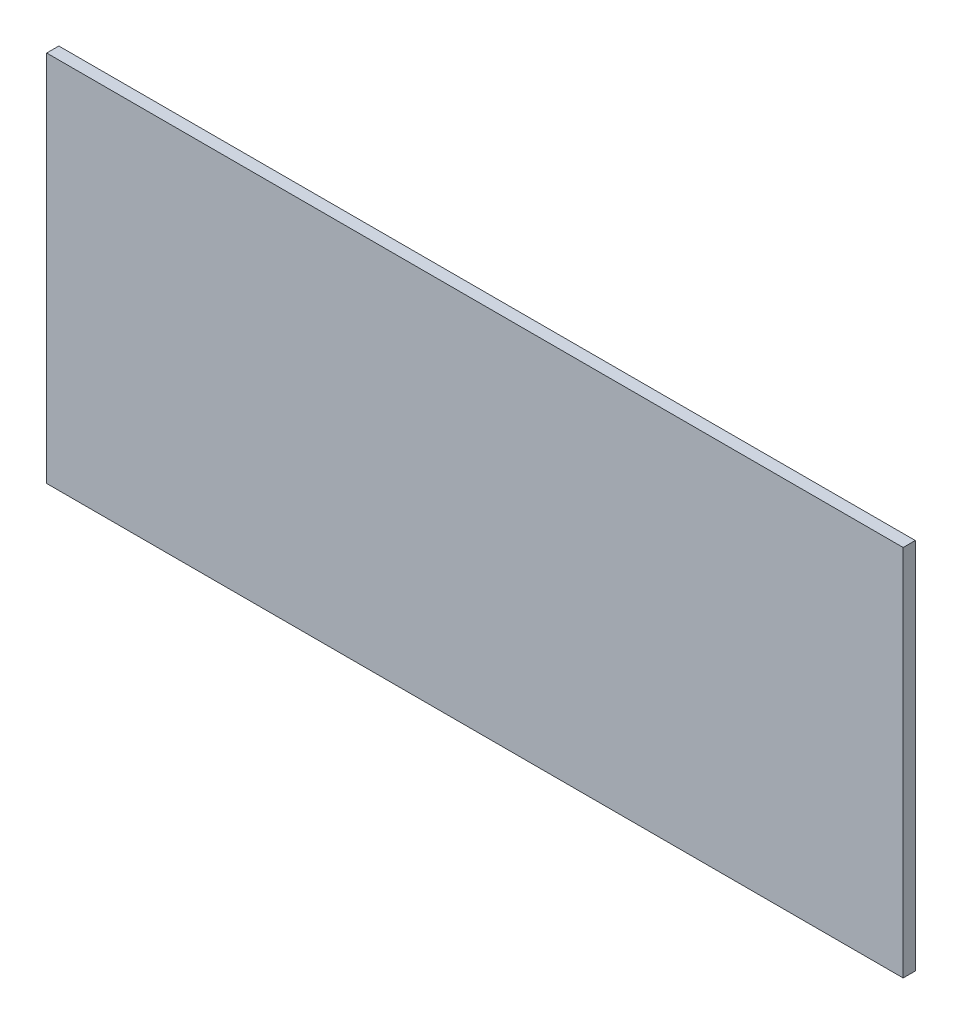
from build123d import *

# Parameters (mm, degrees)
SKETCH1_W           = 2118
SKETCH1_H           = 922
BOSS_EXTRUDE1_DEPTH = 30


with BuildPart() as part:
    # Sketch1 → Boss-Extrude1 (new body)
    with BuildSketch(Plane.XY):
        with Locations((1059, 461)):
            Rectangle(SKETCH1_W, SKETCH1_H)
    extrude(amount=BOSS_EXTRUDE1_DEPTH)


solid = part.part
